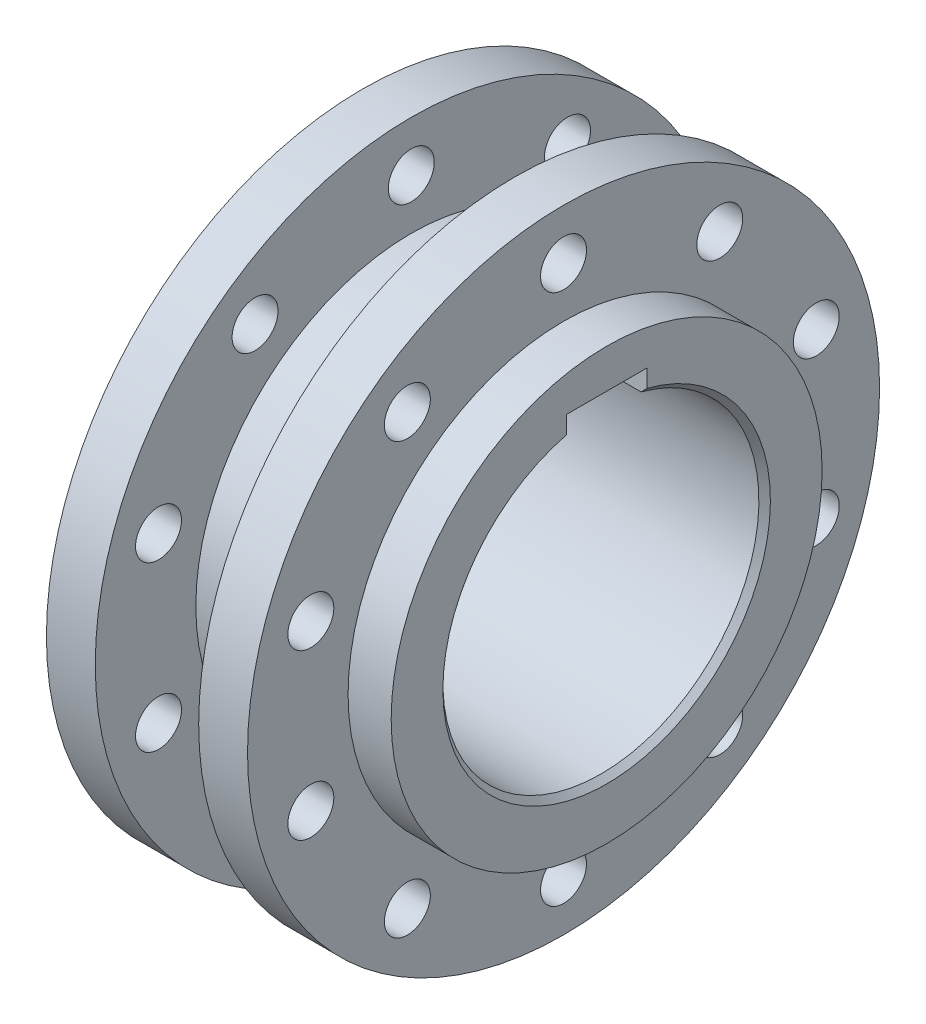
SolidWorks part; units mm, degrees
material "普通碳钢"
ref_plane "Front Plane" through (0, 0, 0) normal (0, 0, 1) x (1, 0, 0)
ref_plane "Top Plane" through (0, 0, 0) normal (0, 1, 0) x (1, 0, 0)
ref_plane "Right Plane" through (0, 0, 0) normal (1, 0, 0) x (0, 0, -1)
sketch "Sketch1" plane through (0, 0, 0) normal (0, 0, 1) x (1, 0, 0)
  line L0 (-50, 57) -> (-50, 75)
  line L1 (55, 0) -> (-55, 0) construction
  line L2 (-50, 75) -> (-35, 75)
  line L3 (-35, 75) -> (-35, 110)
  line L4 (-35, 110) -> (-18, 110)
  line L5 (-18, 110) -> (-18, 75)
  line L6 (-18, 75) -> (18, 75)
  line L7 (0, -55) -> (0, 55) construction
  line L8 (-54.2769, 0) -> (51.2532, 0) construction
  line L9 (0, 60.1733) -> (0, 0) construction
  line L10 (18, 110) -> (18, 75)
  line L11 (35, 110) -> (18, 110)
  line L12 (35, 75) -> (35, 110)
  line L13 (50, 75) -> (35, 75)
  line L14 (50, 57) -> (50, 75)
  line L15 (-48, 55) -> (48, 55)
  line L16 (-48, 55) -> (-50, 57)
  line L17 (48, 55) -> (50, 57)
  point P17 (0, 75)
  point P22 (-50, 55)
  point P23 (50, 55)
  dimension "D1" = 36
  dimension "D2" = 70
  dimension "D3" = 100
  dimension "D4" = 110
  dimension "D5" = 75
  dimension "D6" = 55
revolve "Revolve1" add sketch "Sketch1" angle 360 about L8
sketch "Sketch2" plane through (-35, 0, 0) normal (-1, 0, 0) x (0, 0, 1)
  line L0 (0, -55) -> (0, 55) construction
  circle A0 centre (0, 92.5) radius 8
  circle A1 centre (0, 0) radius 92.5 construction
  dimension "D1" = 185
  dimension "D2" = 16
extrude "Cut-Extrude1" cut sketch "Sketch2" against normal through all
pattern_circular "CirPattern1" count 10 over 360 about axis through (0, 0, 0) along (1, 0, 0) of "Cut-Extrude1"
sketch "Sketch3" plane through (50, 0, 0) normal (1, 0, 0) x (0, 0, -1)
  line L0 (14, 61.4) -> (-14, 61.4)
  line L1 (0, 55) -> (0, -55) construction
  line L2 (-14, 61.4) -> (-14, 0)
  line L3 (55, 0) -> (-55, 0) construction
  line L4 (0, 61.4) -> (0, -61.4) construction
  line L5 (-14, 0) -> (14, 0)
  line L6 (0, 0) -> (-34.1825, 0) construction
  line L7 (14, 61.4) -> (14, 0)
  point P14 (14, 0)
  point P15 (-14, 0)
  dimension "D1" = 28
  dimension "D2" = 61.4
extrude "Cut-Extrude2" cut sketch "Sketch3" against normal through all
